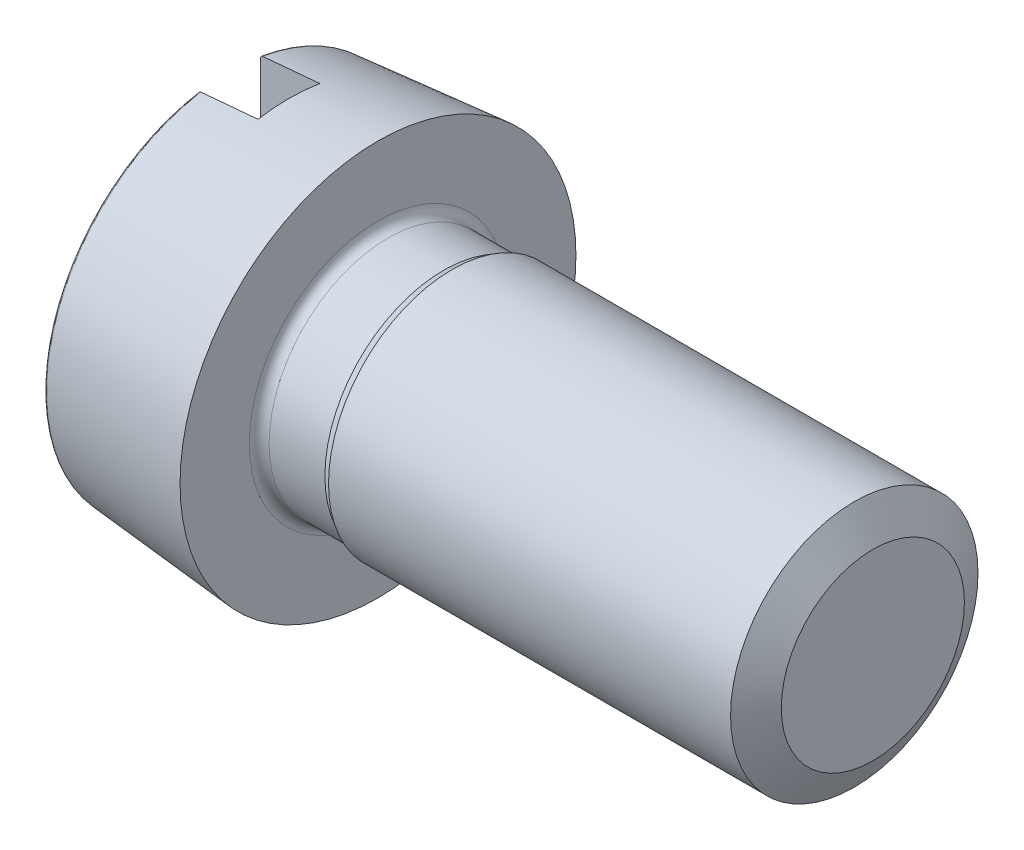
from build123d import *

# Parameters (mm, degrees)
CUT_EXTRUDE_1_DEPTH = 2.4


with BuildPart() as part:
    # 草图1 → Revolve 665 (revolve)
    with BuildSketch(Plane.XY, mode=Mode.PRIVATE) as revolve_665_sk:
        with BuildLine():
            Line((0, 0), (0, 7.383434901))
            ThreePointArc((0, 7.383434901), (0.026272266, 7.450993922), (0.091284426, 7.483054371))
            Line((0.091284426, 7.483054371), (6, 8))
            Line((6, 8), (6, 5.2))
            ThreePointArc((6, 5.2), (6.117157288, 4.917157288), (6.4, 4.8))
            Line((6.4, 4.8), (8.653589838, 4.8))
            Line((8.653589838, 4.8), (9, 5))
            Line((9, 5), (26, 5))
            Line((26, 5), (26, 0))
            Line((26, 0), (0, 0))
        make_face()
    revolve(revolve_665_sk.sketch.rotate(Axis((0, 0, 0), (1, 0, 0)), 90), axis=Axis((0, 0, 0), (1, 0, 0)))

    # 草图2 → 切除-拉伸1 (cut)
    with BuildSketch(Plane.ZY):
        with BuildLine():
            Line((1.25, 7.901740315), (1.25, -7.901740315))
            ThreePointArc((1.25, -7.901740315), (0, -8), (-1.25, -7.901740315))
            Line((-1.25, -7.901740315), (-1.25, 7.901740315))
            ThreePointArc((-1.25, 7.901740315), (0, 8), (1.25, 7.901740315))
        make_face()
    extrude(amount=-CUT_EXTRUDE_1_DEPTH, mode=Mode.SUBTRACT)

    # 草图3 → 切除-旋转1 (revolve, cut)
    with BuildSketch(Plane(origin=(0, 0, 0), x_dir=(1, 0, 0), z_dir=(0, 1, 0)), mode=Mode.PRIVATE) as cut_revolve_1_sk:
        Polygon((25.250022, 5), (26.749978, 5), (26, 3.701), align=None)
    revolve(cut_revolve_1_sk.sketch.rotate(Axis((0, 0, 0), (1, 0, 0)), 180), axis=Axis((0, 0, 0), (1, 0, 0)), mode=Mode.SUBTRACT)


solid = part.part
